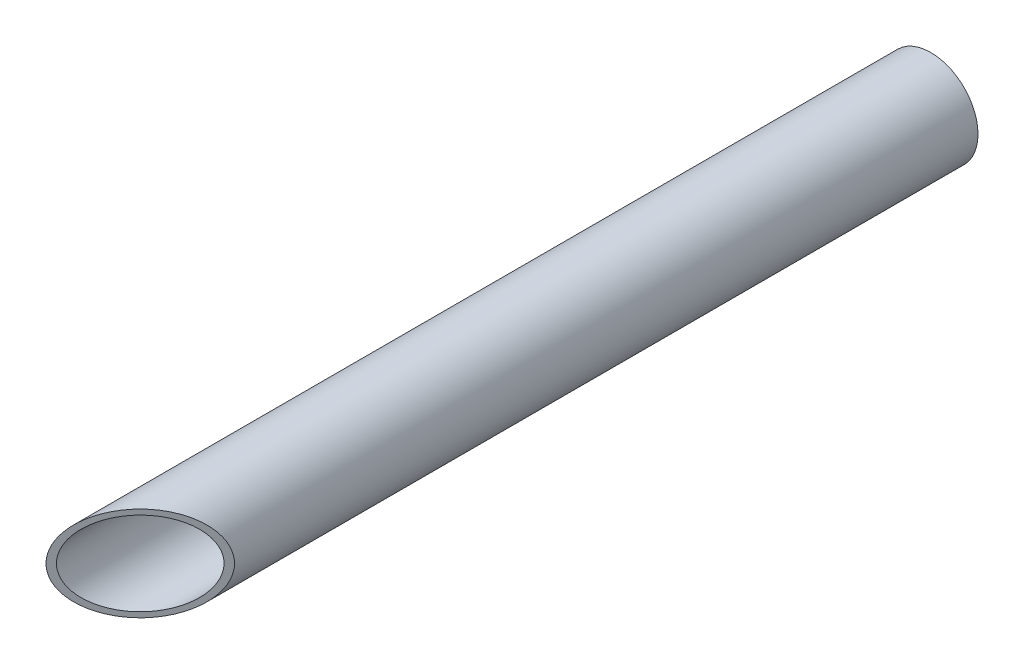
SolidWorks part; units mm, degrees
ref_plane "Front" through (0, 0, 0) normal (0, 0, 1) x (1, 0, 0)
ref_plane "Top" through (0, 0, 0) normal (0, 1, 0) x (1, 0, 0)
ref_plane "Right" through (0, 0, 0) normal (1, 0, 0) x (0, 0, -1)
sketch "Sketch1" plane through (0, 0, 0) normal (0, 0, 1) x (1, 0, 0)
  circle A0 centre (0, 0) radius 9
  circle A1 centre (0, 0) radius 8
  dimension "D1" = 18
  dimension "D2" = 1
extrude "Boss-Extrude1" add sketch "Sketch1" along normal blind 160
sketch "Sketch2" plane through (0, 0, 0) normal (0, 1, 0) x (1, 0, 0)
  line L1 (-9, -160) -> (9, -142)
  line L3 (-9, -160) -> (9, -160)
  line L4 (9, -160) -> (9, -142)
extrude "Cut-Extrude1" cut sketch "Sketch2" against normal mid plane 160
